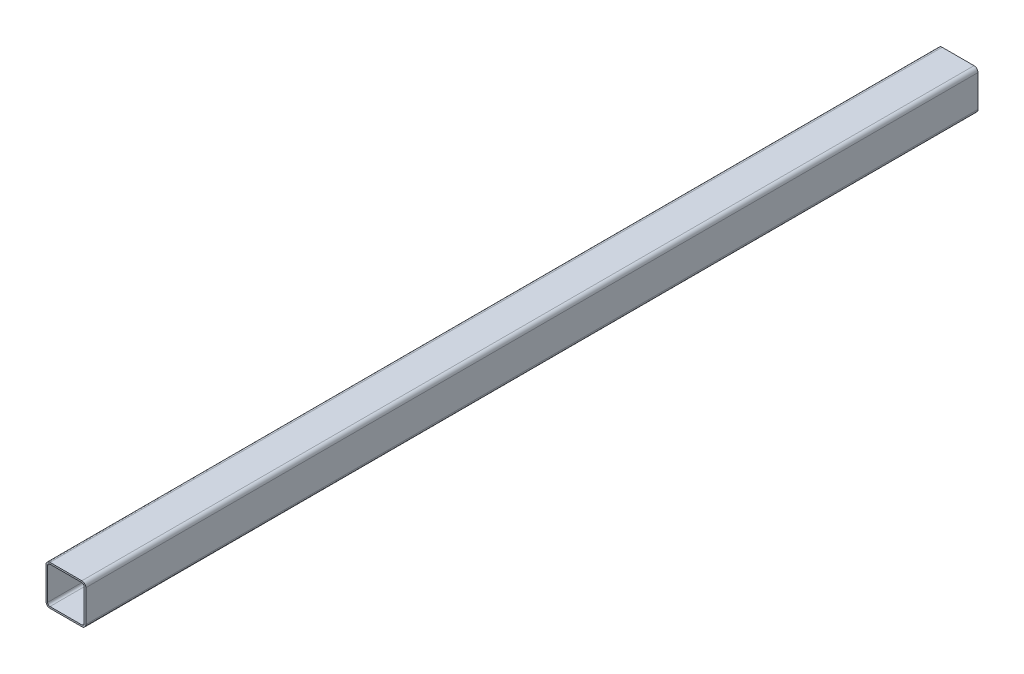
SolidWorks part; units mm, degrees
ref_plane "Front Plane" through (0, 0, 0) normal (0, 0, 1) x (1, 0, 0)
ref_plane "Top Plane" through (0, 0, 0) normal (0, 1, 0) x (1, 0, 0)
ref_plane "Right Plane" through (0, 0, 0) normal (1, 0, 0) x (0, 0, -1)
other "Configuration Table"
sketch "Sketch1" plane through (0, 0, 0) normal (0, 0, 1) x (1, 0, 0)
  line L0 (-92, 80) -> (-92, -80)
  line L1 (-80, 100) -> (80, 100)
  line L2 (-100, 80) -> (-100, -80)
  line L3 (-80, -100) -> (80, -100)
  line L4 (100, 80) -> (100, -80)
  line L5 (-100, 100) -> (100, -100) construction
  line L6 (-100, -100) -> (100, 100) construction
  line L7 (-80, -92) -> (80, -92)
  line L8 (92, 80) -> (92, -80)
  line L9 (-80, 92) -> (80, 92)
  arc A0 (-100, -80) -> (-80, -100) centre (-80, -80) ccw
  arc A1 (80, -100) -> (100, -80) centre (80, -80) ccw
  arc A2 (80, 100) -> (100, 80) centre (80, 80) cw
  arc A3 (-80, 100) -> (-100, 80) centre (-80, 80) ccw
  arc A4 (-92, -80) -> (-80, -92) centre (-80, -80) ccw
  arc A5 (80, -92) -> (92, -80) centre (80, -80) ccw
  arc A6 (80, 92) -> (92, 80) centre (80, 80) cw
  arc A7 (-80, 92) -> (-92, 80) centre (-80, 80) ccw
  point P0 (0, 0)
  dimension "D3" = 20
  dimension "D1" = 200
  dimension "D2" = 200
  dimension "D4" = 8
extrude "Boss-Extrude1" add sketch "Sketch1" along normal blind 4480
